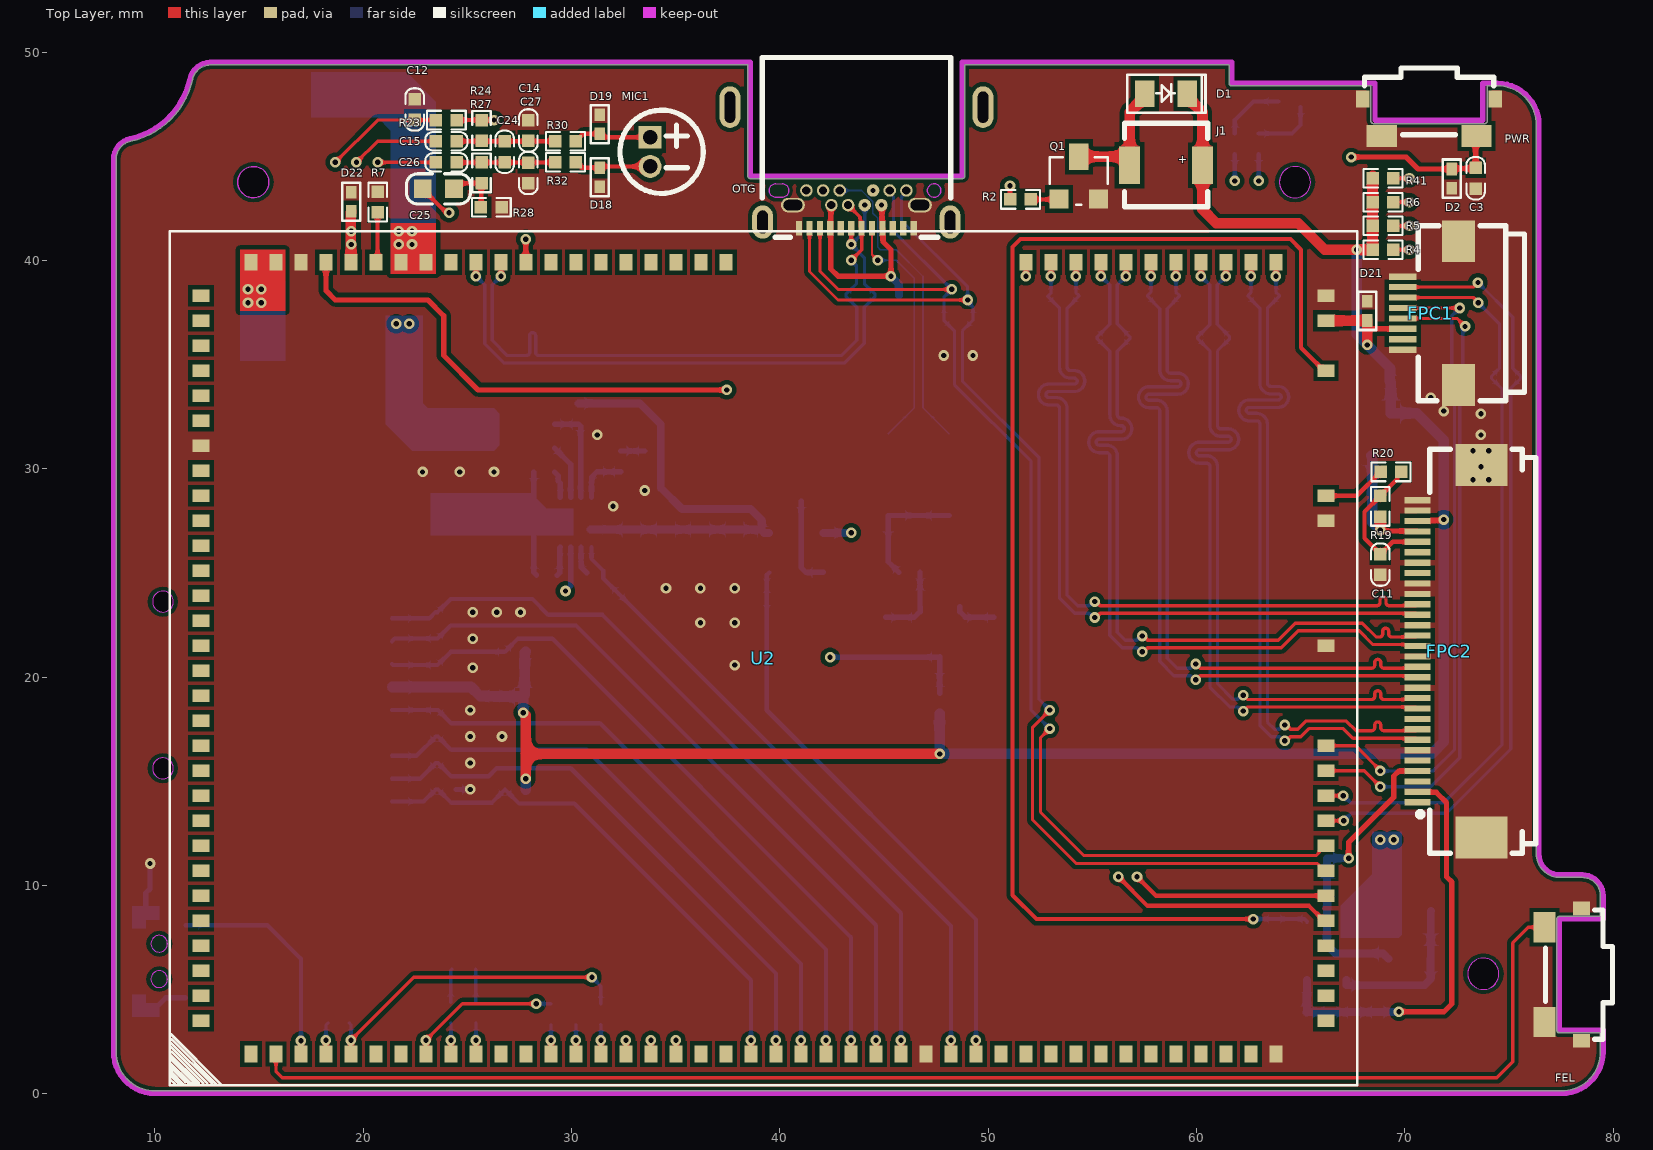
[diagram p0: Top Layer view]
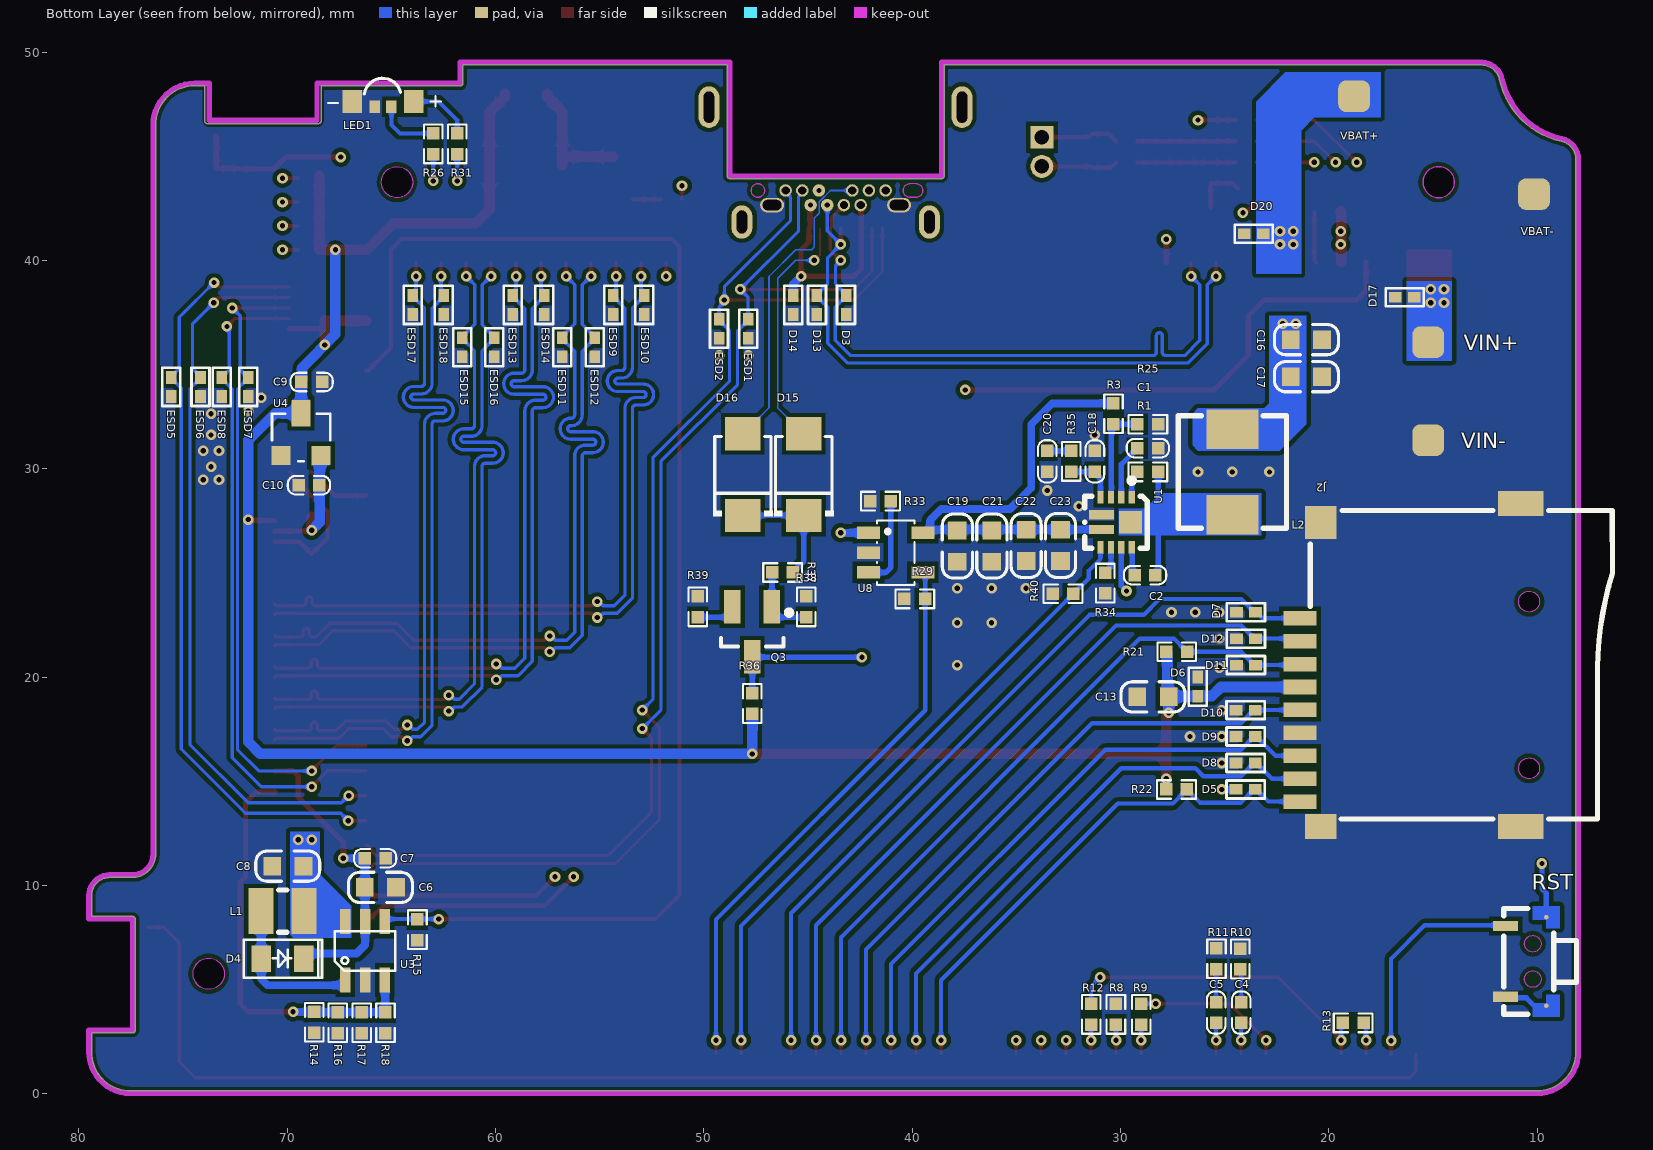
[diagram p1: Bottom Layer view, seen from below]
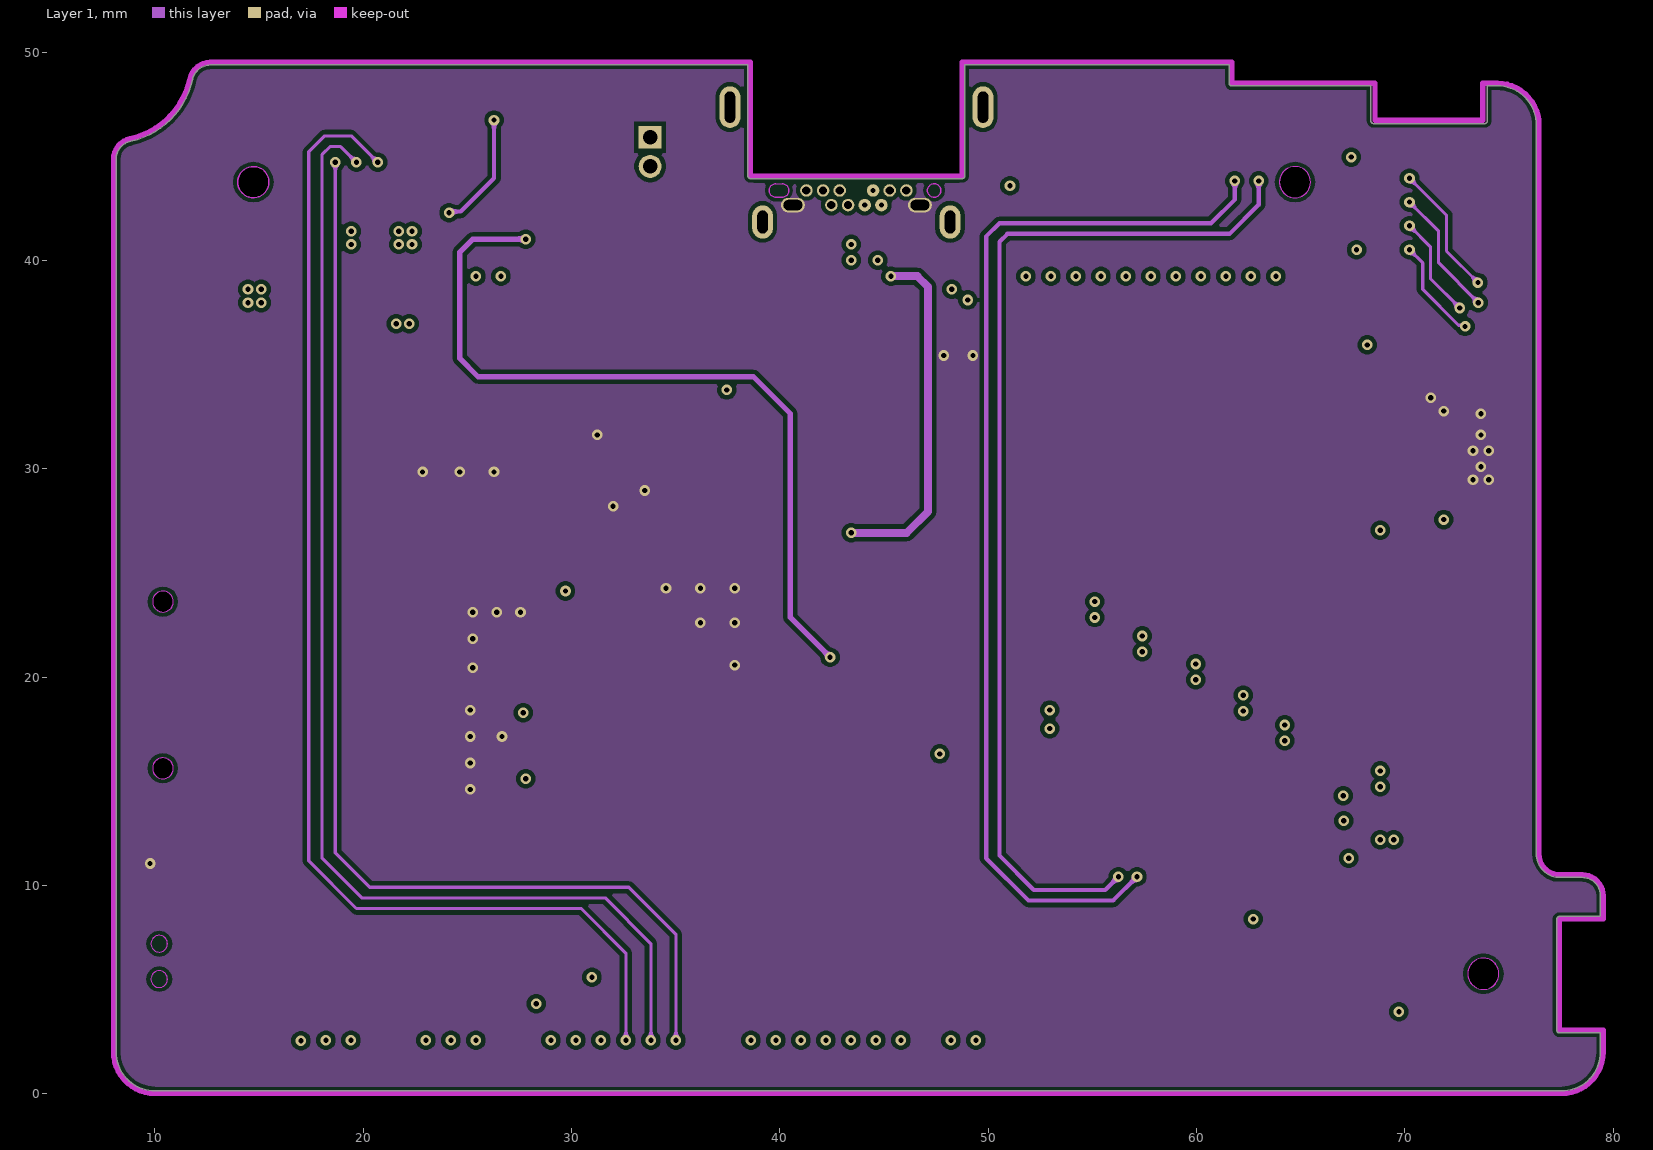
[diagram p2: Layer 1]
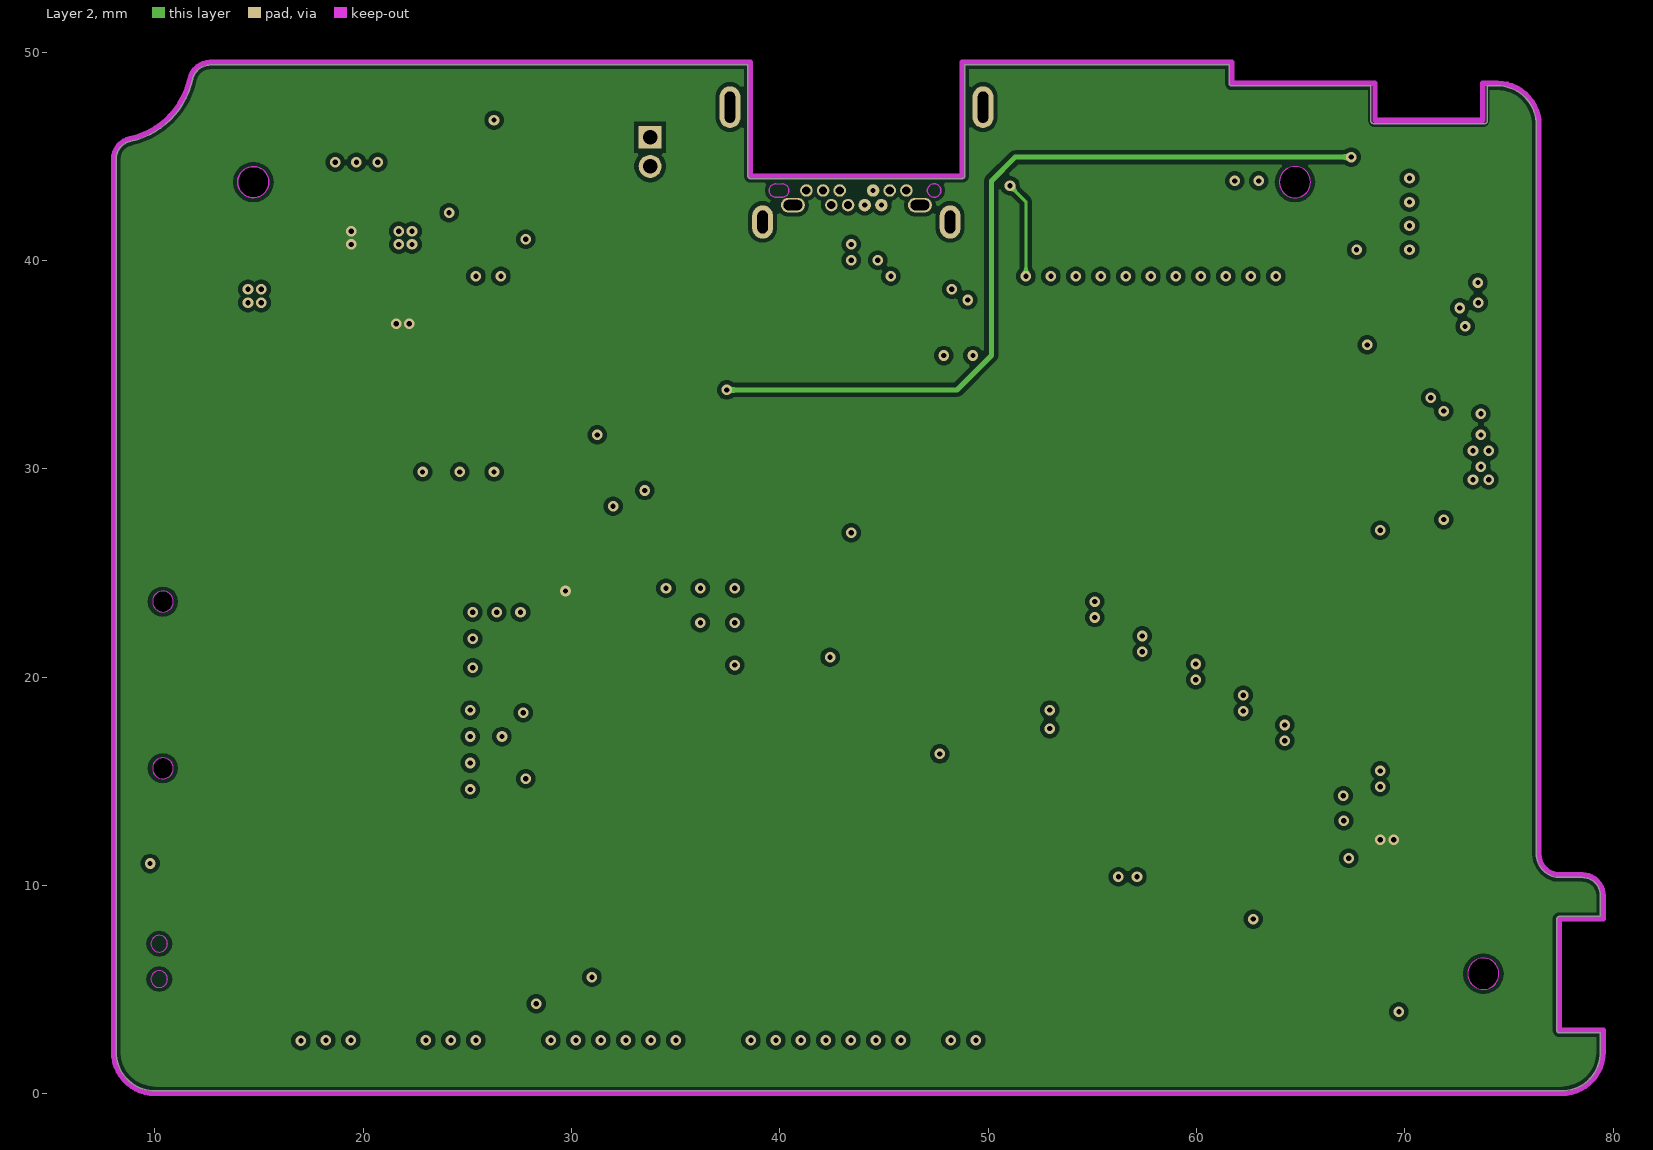
[diagram p3: Layer 2]
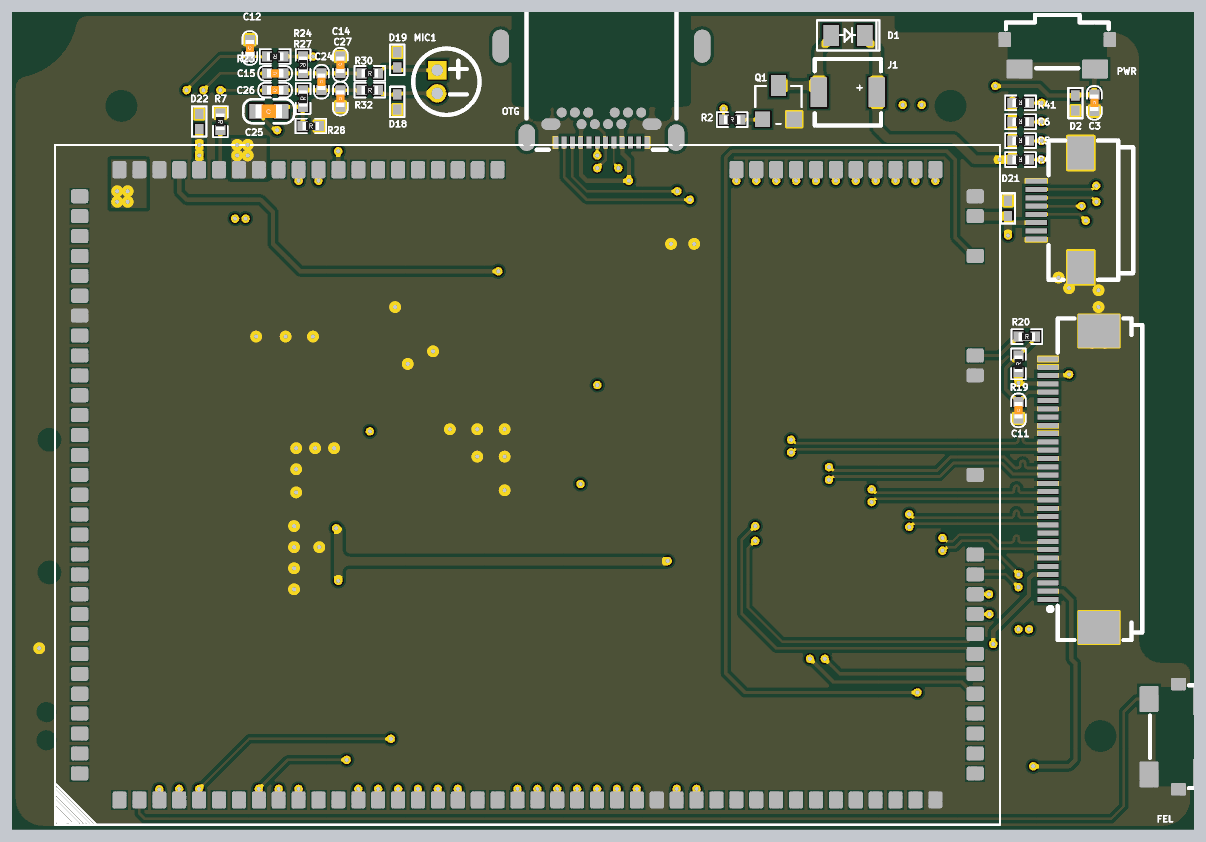
[diagram p4: 3D render of the assembled board from above, using the file's embedded part models]
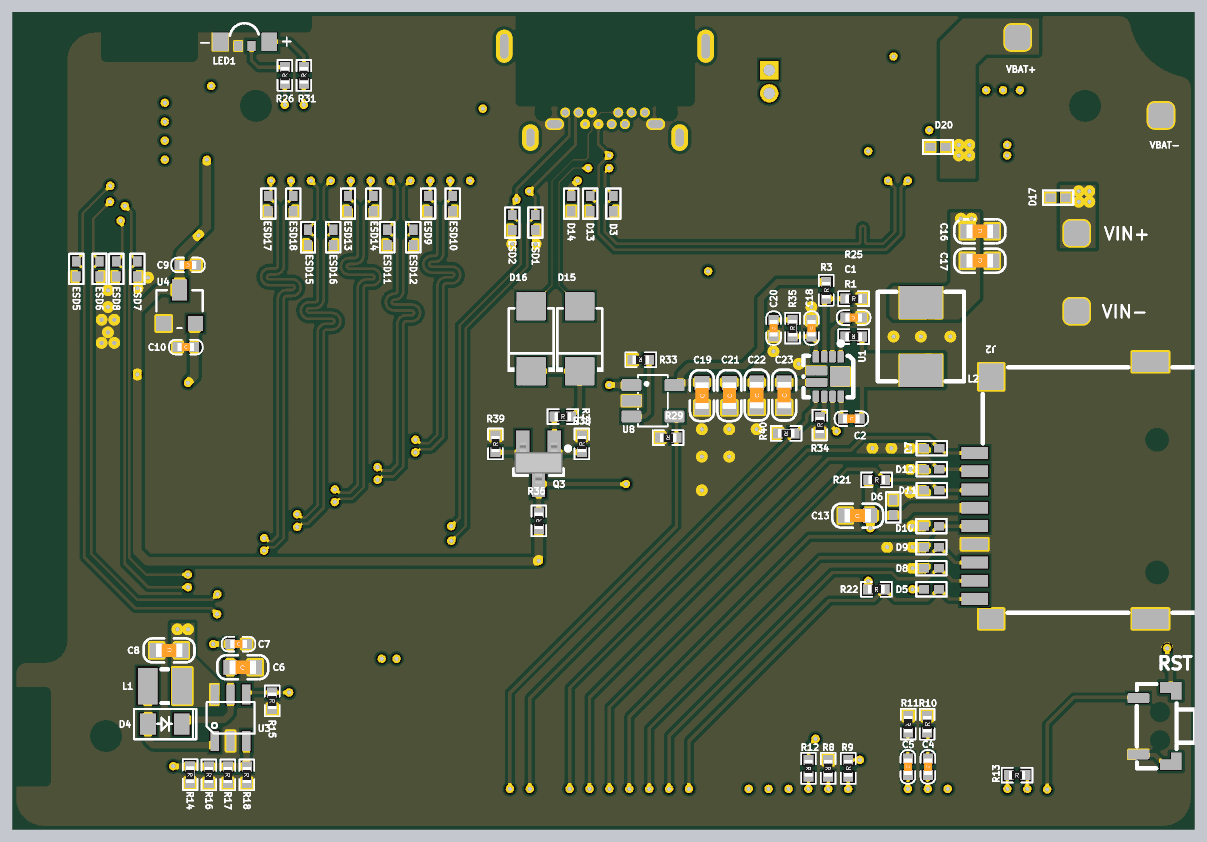
[diagram p5: 3D render of the assembled board from below, using the file's embedded part models]
# Altium PCB MISC105407.PcbDoc (part 1 of 2)
Units mm, origin at the board's own origin, x right, y up, seen from the top; angles counter-clockwise.
Board outline 71.25 x 49.25 mm, 4 copper layers (Top Layer, Layer 1, Layer 2, Bottom Layer), stack 0.603 mm thick; 129 components, 86 nets, 475 pads, 140 vias.

## Layer stack, top to bottom
Top Solder: solder mask 0.0102, Solder Resist, Dk 3.5
Top Layer: signal copper 0.0356
Dielectric 2: prepreg 0.0711, PP-006, Dk 4.1
Layer 1: signal copper 0.035
Dielectric 1: dielectric 0.32, FR-4, Dk 4.8
Layer 2: signal copper 0.035
Dielectric 3: prepreg 0.0711, PP-006, Dk 4.1
Bottom Layer: signal copper 0.0356
Bottom Solder: solder mask 0.0102, Solder Resist, Dk 3.5

## Board outline
8.154,2.006 ccw(c10.026,2.006) 10.026,0.134 77.526,0.134 ccw(c77.526,2.006) 79.399,2.006 79.399,2.921 77.43,2.921 cw(c77.43,3.048) 77.303,3.048 77.303,8.382 cw(c77.43,8.382) 77.43,8.509 79.399,8.509 79.399,9.506 ccw(c78.526,9.506) 78.526,10.379 77.446,10.379 cw(c77.446,11.506) 76.319,11.506 76.319,46.506 ccw(c74.446,46.506) 74.446,48.379 cw(c74.446,48.507) 74.445,48.379 73.965,48.379 73.965,46.696 cw(c73.838,46.696) 73.838,46.569 68.504,46.569 cw(c68.504,46.696) 68.376,46.696 68.376,48.379 61.696,48.379 cw(c61.696,48.506) 61.569,48.506 61.569,49.379 48.889,49.379 48.889,44.055 cw(c48.761,44.055) 48.761,43.927 48.606,43.927 cw(c48.538,44.035) 48.538,43.908 38.838,43.908 cw(c38.838,44.035) 38.77,43.927 38.601,43.927 cw(c38.601,44.055) 38.474,44.055 38.474,49.379 12.67,49.379 ccw(c12.67,53.145) 12.671,49.379 12.67,49.379 ccw(c12.67,48.506) 11.817,48.69 cw(c8.027,49.506) 8.843,45.716 cw(c8.596,46.862) 8.843,45.716 ccw(c8.827,45.791) 8.843,45.716 ccw(c9.027,44.862) 8.154,44.863
cut-out: 73.026,5.756 ccw(c73.776,5.756) 73.776,5.006 ccw(c73.776,5.756) 74.526,5.756 ccw(c73.776,5.756) 73.776,6.506 ccw(c73.776,5.756)
cut-out: 63.986,43.756 ccw(c64.736,43.756) 64.736,43.006 ccw(c64.736,43.756) 65.486,43.756 ccw(c64.736,43.756) 64.736,44.506 ccw(c64.736,43.756)
cut-out: 14.736,43.006 cw(c14.736,43.756) 13.986,43.756 cw(c14.736,43.756) 14.736,44.506 cw(c14.736,43.756) 15.486,43.756 cw(c14.736,43.756)

## Design rules (kind name [scope] priority, off if disabled: settings)
Clearance [All] p1: gap=0.051 ignorepadtopadclearanceinfootprint=FALSE except(0.203: Arc-Poly Track-Poly SMDPad-Poly THPad-Poly Via-Poly Fill-Poly Poly-Poly Poly-Region Poly-Text Poly-Hole)
ComponentClearance [All] p1: gap=0 collisioncheckmode=3 verticalgap=0 showdistances=FALSE
DiffPairsRouting [InDifferentialPairClass('D_90om')] p1: maxlimit=0.254 minlimit=0.203 mostfreqgap=0.203 toplayer_minwidth=0.158 toplayer_maxwidth=0.158 toplayer_prefwidth=0.158 midlayer1_minwidth=0.158 midlayer1_maxwidth=0.158 midlayer1_prefwidth=0.158 midlayer2_minwidth=0.158 midlayer2_maxwidth=0.158 midlayer2_prefwidth=0.158 bottomlayer_minwidth=0.158 bottomlayer_maxwidth=0.158 bottomlayer_prefwidth=0.158 maxuncoupledlength=12.7
MinimumSolderMaskSliver [All] p1: minsoldermaskwidth=0
PolygonConnect [All] p1: connectstyle=Direct reliefconductorwidth=0.254 reliefentries=4 polygonreliefangle="90 Angle" airgapwidth=0.254
RoutingVias [All] p1: holewidth=0.254 width=0.508 viastyle="Through Hole" minholewidth=0.254 minwidth=0.508 maxholewidth=0.254 maxwidth=0.508
SilkToSilkClearance [All] p1: silktosilkclearance=0
SilkToSolderMaskClearance [IsPad] p1: minsilkscreentomaskgap=0 clearancetoexposedcopper=TRUE
SolderMaskExpansion [All] p1: expansion=0.102 istentingtop=FALSE
Width [All] p1: maxlimit=1.27 minlimit=0.025 preferedwidth=0.254
25 further rules are at their usual default settings.

## Classes and differential pairs
differential pair class D_90om: MICIN1 MIPI_CL MIPI_D0 MIPI_D1 MIPI_D2 MIPI_D3 USB0
differential pair MICIN1: +MICIN1_P -MICIN1_N
differential pair MIPI_D3: +MIPI_D3_P -MIPI_D3_N
differential pair MIPI_D2: +MIPI_D2_P -MIPI_D2_N
differential pair MIPI_D1: +MIPI_D1_P -MIPI_D1_N
differential pair MIPI_CL: +MIPI_CL_P -MIPI_CL_N
differential pair USB0: +USB0_P -USB0_N
differential pair MIPI_D0: +MIPI_D0_P -MIPI_D0_N

## Components (designator, comment, footprint, x,y, rotation, side; value= is the part's Value field where it differs from the comment)
C1 "C-16-225(±10%)" C0402 28.694,30.988 r180 bottom
C2 "C-50-104(±10%)" C0402 28.829,24.892 r0 bottom
C3 "C-25-104" C0402 73.406,43.942 r90 top
C4 "C-25-104" C0402 24.212,3.896 r270 bottom
C5 "C-25-104" C0402 25.418,3.896 r270 bottom
C6 "C-25-106" C0603 65.532,9.906 r180 bottom
C7 "C-25-104" C0402 65.786,11.303 r0 bottom
C8 "C-25-106" C0603 69.977,10.922 r0 bottom
C9 "C-25-104" C0402 68.834,34.163 r180 bottom
C10 "C-25-104" C0402 68.961,29.21 r0 bottom
C11 "C-25-104" C0402 68.834,25.4 r270 top
C12 "C-50-105" C0402 22.479,47.244 r270 top
C13 "C-25-106" C0603 28.448,19.05 r180 bottom
C14 "C-50-330" C0402 27.94,46.236 r270 top
C15 "C-50-104" C0402 24.003,45.72 r0 top
C16 "C-16-106(±10%)" C0603 21.082,36.195 r0 bottom
C17 "C-16-106(±10%)" C0603 21.082,34.417 r0 bottom
C18 "C-50-472(±10%)" C0402 31.234,30.353 r270 bottom
C19 "C-16-106(±10%)" C0603 37.838,26.289 r90 bottom
C20 "C-50-220(±10%)" C0402 33.52,30.353 r90 bottom
C21 "C-16-106(±10%)" C0603 36.187,26.289 r90 bottom
C22 "C-16-106(±10%)" C0603 34.536,26.32 r90 bottom
C23 "C-16-106(±10%)" C0603 32.885,26.32 r90 bottom
C24 "C-50-101" C0402 26.797,45.212 r90 top
C25 "C-50-106" C0603 23.622,43.434 r0 top
C26 "C-50-104" C0402 24.003,44.704 r0 top
C27 "C-50-330" C0402 27.94,44.196 r90 top
D1 "1N5819" SOD323 58.547,48.006 r0 top
D2 "AU0511P1" ESD0402A 72.263,43.942 r90 top
D3 "AU0511P1" ESD0402A 43.18,37.846 r270 bottom
D4 "1N5819" SOD323 70.231,6.477 r180 bottom
D5 "AU0511P1" ESD0402A 24.019,14.604 r0 bottom
D6 "AU0511P1" ESD0402A 26.305,19.557 r90 bottom
D7 "AU0511P1" ESD0402A 24.003,23.114 r0 bottom
D8 "AU0511P1" ESD0402A 24.019,15.874 r0 bottom
D9 "AU0511P1" ESD0402A 24.019,17.144 r0 bottom
D10 "AU0511P1" ESD0402A 24.019,18.414 r0 bottom
D11 "AU0511P1" ESD0402A 24.003,20.574 r0 bottom
D12 "AU0511P1" ESD0402A 24.003,21.844 r0 bottom
D13 "AU0511P1" ESD0402A 44.577,37.846 r270 bottom
D14 "AU0511P1" ESD0402A 45.72,37.846 r270 bottom
D15 "SS34F_C18199199" SMAF_L3.5-W2.6-LS4.7-RD-1 45.212,29.718 r90 bottom
D16 "SS34F_C18199199" SMAF_L3.5-W2.6-LS4.7-RD-1 48.133,29.718 r90 bottom
D17 "AU0511P1" ESD0402A 16.383,38.227 r0 bottom
D18 "AU0511P1" ESD0402A 31.368,44.009 r90 top
D19 "AU0511P1" ESD0402A 31.37,46.517 r270 top
D20 "AU0511P1" ESD0402A 23.622,41.275 r0 bottom
D21 "AU0511P1" ESD0402A 68.199,37.592 r90 top
D22 "AU0511P1" ESD0402A 19.431,42.799 r270 top
ESD1 "AU0511P1" ESD0402A 47.879,36.703 r270 bottom
ESD2 "AU0511P1" ESD0402A 49.276,36.703 r270 bottom
ESD5 "AU0511P1" ESD0402A 75.565,33.909 r270 bottom
ESD6 "AU0511P1" ESD0402A 74.168,33.909 r270 bottom
ESD7 "AU0511P1" ESD0402A 71.882,33.909 r270 bottom
ESD8 "AU0511P1" ESD0402A 73.152,33.909 r270 bottom
ESD9 "AU0511P1" ESD0402A 54.356,37.846 r270 bottom
ESD10 "AU0511P1" ESD0402A 52.873,37.846 r270 bottom
ESD11 "AU0511P1" ESD0402A 56.81,35.814 r270 bottom
ESD12 "AU0511P1" ESD0402A 55.245,35.814 r270 bottom
ESD13 "AU0511P1" ESD0402A 59.182,37.846 r270 bottom
ESD14 "AU0511P1" ESD0402A 57.658,37.846 r270 bottom
ESD15 "AU0511P1" ESD0402A 61.595,35.814 r270 bottom
ESD16 "AU0511P1" ESD0402A 60.071,35.814 r270 bottom
ESD17 "AU0511P1" ESD0402A 63.982,37.846 r270 bottom
ESD18 "AU0511P1" ESD0402A 62.484,37.846 r270 bottom
FEL "TSB017A3126A02" KEY-SMD_YTSB017A0312502B#1 77.597,5.715 r90 top
FPC1 "AFC01-S08FCA-00" FPC-SMD_P0.50-8P_FGS-XJ-H2.0 71.247,37.465 r270 top locked
FPC2 "FPC-05F-30PH20" FPC-SMD_30P-P0.50_XUNPU_FPC-05F-30PH20 72.147,21.241 r90 top locked
J1 "FUET-4020" BUZ-SMD_L4.0-W4.0-P3.50-L 58.547,44.577 r180 top
J2 "TF-115-BCP9" TF-SMD_TF-115-BCP9 16.095,20.571 r90 bottom locked
L1 "10uH" IND-SMD_L2.5-W2.0 70.231,8.763 r180 bottom
L2 "FXL0518-2R2-M" IND-SMD_L5.2-W5.4 24.638,29.845 r270 bottom
LED1 "XL-3210SURUGC" LED-SMD_4P-L3.2-W1.5_HTG-3210SURUBGC 65.405,47.498 r180 bottom
MIC1 "GMI4015P-2C-64db" MIC-TH_BD4.0-P1.40-D0.4-L-FD 33.782,45.212 r270 top
OTG "GT-USB-9009B" USB-C-SMD_GT-USB-9009B 43.688,44.45 r180 top (schematic designator USBC1)
PWR "TSB017A3126A02" KEY-SMD_YTSB017A0312502B#2 71.171,46.863 r180 top
Q1 "S9013" SOT23 54.356,43.942 r0 top
Q3 "8050-S" SOT-23-3 46.741,23.368 r270 bottom
R1 "R-304J" R0402 28.694,29.845 r0 bottom
R2 "R-152J" R0402 51.562,42.926 r0 top
R3 "R-304F" R0402 30.345,32.639 r90 bottom
R4 "R-472J" R0402 68.961,40.513 r180 top
R5 "R-472J" R0402 68.961,41.656 r180 top
R6 "R-472J" R0402 68.961,42.799 r180 top
R7 "R-103J" R0402 20.701,42.799 r270 top
R8 "R-0J" R0402 30.226,3.81 r270 bottom
R9 "R-202J" R0402 29.019,3.81 r90 bottom
R10 "R-220J" R0402 24.257,6.469 r90 bottom
R11 "R-220J" R0402 25.4,6.477 r270 bottom
R12 "R-105J" R0402 31.414,3.81 r270 bottom
R13 "R-104J" R0402 18.84,3.397 r180 bottom
R14 "NC" R0402 68.707,3.429 r270 bottom
R15 "1M" R0402 63.754,7.874 r270 bottom
R16 "8R2" R0402 67.574,3.408 r270 bottom
R17 "8R2" R0402 66.431,3.408 r270 bottom
R18 "8R2" R0402 65.288,3.408 r270 bottom
R19 "R-103J" R0402 68.834,28.194 r90 top
R20 "R-0J" R0402 69.342,29.845 r0 top
R21 "R-103J" R0402 27.305,21.209 r180 bottom
R22 "R-103J" R0402 27.321,14.604 r180 bottom
R23 "R-102" R0402 24.003,46.736 r180 top
R24 "R-152" R0402 25.689,46.236 r270 top
R25 "R-104F" R0402 28.694,32.131 r180 bottom
R26 "R-202J" R0402 62.992,45.593 r90 bottom
R27 "R-152" R0402 25.689,44.2 r90 top
R28 "R-102" R0402 26.162,42.545 r0 top
R29 "R-103J" R0402 39.878,23.749 r0 bottom
R30 "R-104F" R0402 29.718,45.72 r0 top
R31 "R-202J" R0402 61.849,45.593 r90 bottom
R32 "R-304F" R0402 29.718,44.704 r0 top
R33 "R-332J" R0402 41.529,28.448 r0 bottom
R34 "R-154J" R0402 30.734,24.511 r90 bottom
R35 "R-622F" R0402 32.377,30.353 r90 bottom
R36 "R-103J" R0402 47.678,18.729 r90 bottom
R37 "R-103J" R0402 46.228,25.019 r180 bottom
R38 "R-103J" R0402 45.085,23.368 r90 bottom
R39 "R-5R0J" R0402 50.292,23.368 r90 bottom
R40 "R-103J" R0402 32.766,24.003 r0 bottom
R41 "R-472J" R0402 68.961,43.942 r180 top
RST "LXTD-0204-034" SW-SMD_LXTD-0204-034 10.541,6.35 r90 bottom
U1 "TPS61089RNRR" VQFN-HR_L2.5-W2.0-P0.50-TL-EP 30.218,27.432 r270 bottom
U2 "HelperA133Core" "A133 - duplicate" 10.743,0.385 r90 top locked
U3 "HM5663" SOT23-6 66.04,6.858 r270 bottom
U4 "xc6206p182mr" SOT23 69.342,31.623 r180 bottom
U8 "MT9700" SOT-23-5_L3.0-W1.7-P0.95-LS2.8-BR 40.797,25.974 r0 bottom
VBAT+ "Header 1" HDR-LI-1P 18.796,47.879 r90 bottom
VBAT- "Header 1" HDR-LI-1P 10.16,43.18 r90 bottom
VIN+ "Header 1" HDR-LI-1P 15.24,36.068 r90 bottom
VIN- "Header 1" HDR-LI-1P 15.24,31.369 r90 bottom

## Footprints (in the part's own frame and the unit in brackets; to place one, negate y for a bottom-side part, rotate by r counter-clockwise, add the part's x,y. Pads: shape width x height; smd on the part's side, far side on the other; paste and mask are expansions set on the pad)
"A133 - duplicate" [mil]
  rect 31.5x24 smd paste+4.73: 1(59.83,-152.68) 2(59.83,-199.92) 3(59.83,-247.17) 4(59.83,-294.41) 5(59.83,-341.65) 6(59.83,-388.9) 7(59.83,-436.14) 8(59.83,-483.39) 9(59.83,-530.63) 10(59.83,-577.87) 11(59.83,-625.12) 12(59.83,-672.36) 13(59.83,-719.61) 14(59.83,-766.85) 15(59.83,-814.09) 16(59.83,-861.34) 17(59.83,-908.58) 18(59.83,-955.83) 19(59.83,-1003.07) 20(59.83,-1050.32) 21(59.83,-1097.56) 22(59.83,-1144.8) 23(59.83,-1192.05) 24(59.83,-1239.29) 25(59.83,-1286.54) 26(59.83,-1333.78) 27(59.83,-1381.02) 28(59.83,-1428.27) 29(59.83,-1475.51) 30(59.83,-1522.76) 31(59.83,-1570) 32(59.83,-1617.24) 33(59.83,-1664.49) 34(59.83,-1711.73) 35(59.83,-1758.98) 36(59.83,-1806.22) 37(59.83,-1853.46) 38(59.83,-1900.71) 39(59.83,-1947.95) 40(59.83,-1995.2) 41(59.83,-2042.44) 42(59.83,-2089.68) 73(1555.89,-2089.68) 74(1555.89,-2042.44) 75(1555.89,-1995.2) 76(1555.89,-1947.95) 77(1555.89,-1900.71) 78(1555.89,-1853.46) 79(1555.89,-1806.22) 80(1555.89,-1758.98) 81(1555.89,-1711.73) 82(1555.89,-1664.49) 83(1555.89,-1617.24) 95(1555.89,-1050.32) 96(1555.89,-1003.07) 97(1555.89,-955.83) 98(1555.89,-908.58) 99(1555.89,-861.34) 100(1555.89,-814.09) 101(1555.89,-766.85) 102(1555.89,-719.61) 103(1555.89,-672.36) 104(1555.89,-625.12) 105(1555.89,-577.87) 106(1555.89,-530.63) 107(1555.89,-483.39) 108(1555.89,-436.14) 109(1555.89,-388.9) 110(1555.89,-341.65) 111(1555.89,-294.41) 112(1555.89,-247.17) 113(1555.89,-199.92) 114(1555.89,-152.68)
  rect 24x31.5 smd paste+4.73: 43(122.82,-2184.17) 44(170.06,-2184.17) 45(217.31,-2184.17) 46(264.55,-2184.17) 47(311.8,-2184.17) 48(359.04,-2184.17) 49(406.28,-2184.17) 50(453.53,-2184.17) 51(500.77,-2184.17) 52(548.02,-2184.17) 53(595.26,-2184.17) 54(642.5,-2184.17) 58(831.48,-2184.17) 63(1067.7,-2184.17) 64(1114.94,-2184.17) 69(1351.17,-2184.17) 71(1445.65,-2184.17) 72(1492.9,-2184.17) 115(1492.9,-58.19) 116(1445.65,-58.19) 117(1398.41,-58.19) 118(1351.17,-58.19) 119(1303.92,-58.19) 120(1256.68,-58.19) 121(1209.43,-58.19) 122(1162.19,-58.19) 123(1114.94,-58.19) 124(1067.7,-58.19) 125(1020.46,-58.19) 126(973.21,-58.19) 127(925.97,-58.19) 128(878.72,-58.19) 129(831.48,-58.19) 130(784.24,-58.19) 131(736.99,-58.19) 132(689.75,-58.19) 133(642.5,-58.19) 134(595.26,-58.19) 135(548.02,-58.19) 136(500.77,-58.19) 137(453.53,-58.19) 138(406.28,-58.19) 139(359.04,-58.19) 140(311.8,-58.19) 141(264.55,-58.19) 142(217.31,-58.19) 143(170.06,-58.19) 144(122.82,-58.19)
  silkscreen extent 1,-2243 1615,1
BUZ-SMD_L4.0-W4.0-P3.50-L [mm]
  rect 1x1.8 smd: 1(-1.75,0) 2(1.75,0)
  silkscreen extent -2,-2 2,2
C0402 [mm]
  rect 0.6x0.6 smd: 1(0.5,0) 2(-0.5,0)
  silkscreen extent -1.02,-0.44 1.02,0.44, body extent -0.5,-0.25 0.5,0.25, height 0.49
C0603 [mm]
  rect 0.85x0.9 smd: 1(-0.75,0) 2(0.75,0)
  silkscreen extent -1.54,-0.72 1.54,0.72, body extent -0.8,-0.41 0.8,0.4, height 0.88
ESD0402A [mil]
  rect 24x20 smd: 1(-18.63,-0.06) 2(17.37,-0.06)
  silkscreen extent -37,-17 35,17
FPC-SMD_30P-P0.50_XUNPU_FPC-05F-30PH20 [mm]
  rect 0.3x1.25 smd paste+0 mask+0.05: 1(-7.25,1.538) 2(-6.75,1.538) 3(-6.25,1.538) 4(-5.75,1.538) 5(-5.25,1.538) 6(-4.75,1.538) 7(-4.25,1.538) 8(-3.75,1.538) 9(-3.25,1.538) 10(-2.75,1.538) 11(-2.25,1.538) 12(-1.75,1.538) 13(-1.25,1.538) 14(-0.75,1.538) 15(-0.25,1.538) 16(0.25,1.538) 17(0.75,1.538) 18(1.25,1.538) 19(1.75,1.538) 20(2.25,1.538) 21(2.75,1.538) 22(3.25,1.538) 23(3.75,1.538) 24(4.25,1.538) 25(4.75,1.538) 26(5.25,1.538) 27(5.75,1.538) 28(6.25,1.538) 29(6.75,1.538) 30(7.25,1.538)
  rect 2x2.5 smd paste+0 mask+0.05: 31(8.94,-1.538) 32(-8.94,-1.538)
  silkscreen extent -9.7,-4.15 9.7,1.53
FPC-SMD_P0.50-8P_FGS-XJ-H2.0 [mm]
  rect 0.3x1.3 smd paste+0 mask+0.05: 1(1.75,-1.34) 2(1.25,-1.34) 3(0.75,-1.34) 4(0.25,-1.34) 5(-0.25,-1.34) 6(-0.75,-1.34) 7(-1.252,-1.338) 8(-1.75,-1.34)
  rect 2x1.6 smd: 9(3.45,1.34) 10(-3.45,1.34)
  silkscreen extent -4.2,-0.6 4.2,4.5
HDR-LI-1P [mil]
  rrect50% 60x60 smd: 1(0,0)
IND-SMD_L2.5-W2.0 [mm]
  rect 1.2x2.2 smd: 1(1.028,0) 2(-1.028,0)
  silkscreen extent -0.2,-1.02 0.2,1.02
IND-SMD_L5.2-W5.4 [mm]
  rect 1.9x2.5 smd paste+0.051: 1(-2.05,0) 2(2.05,0)
  silkscreen extent -2.7,-2.6 2.7,2.6
KEY-SMD_YTSB017A0312502B#1 [mm]
  rect 1.45x1.05 smd paste+0.051 mask+0: 1(-2.275,0.887) 2(2.275,0.887)
  rect 0.65x0.8 smd paste+0.051 mask+0: 3(-3.175,-0.887) 4(3.175,-0.887)
  Keep-Out Layer lines w0.254: -2.667,0.167 2.667,0.167 ; -2.667,0.167 -2.667,-1.93 -2.667,0.167 ; -2.667,0.167 2.667,0.167 ; 2.667,0.167 2.667,-1.93 2.667,0.167
  silkscreen extent -3.1,-2.38 3.1,0.84
KEY-SMD_YTSB017A0312502B#2 [mm]
  rect 1.45x1.05 smd paste+0.051 mask+0: 1(-2.275,0.887) 2(2.275,0.887)
  rect 0.65x0.8 smd paste+0.051 mask+0: 3(-3.175,-0.887) 4(3.175,-0.887)
  silkscreen extent -3.1,-2.38 3.1,0.84
LED-SMD_4P-L3.2-W1.5_HTG-3210SURUBGC [mm]
  rect 0.5x0.6 smd paste+0 mask+0.05: 1(0.4,-0.132) 2(-0.4,-0.132)
  rect 0.95x1.1 smd paste+0 mask+0.05: 3(1.475,0.132) 4(-1.475,0.132)
  silkscreen extent -2.64,-0.12 2.77,1.24
MIC-TH_BD4.0-P1.40-D0.4-L-FD [mm]
  rect 1.1x1.1 hole 0.7 paste+0.051: 1(-0.7,0)
  round 1.1 hole 0.7 paste+0.051: 2(0.7,0)
  silkscreen extent -2,-1.45 2,2.55
R0402 [mm] "Chip Capacitor; Body 1.0 x 0.5 mm (LxW typ)"
  rect 0.6x0.6 smd: 1(-0.5,0) 2(0.5,0)
  silkscreen extent -0.93,-0.44 0.93,0.44, body extent -0.5,-0.25 0.5,0.25, height 0.38
SMAF_L3.5-W2.6-LS4.7-RD-1 [mm]
  rect 1.6x1.7 smd paste+0.051: 1(-1.96,0) 2(1.96,0)
  silkscreen extent -2.01,-1.43 1.83,1.42
SOD323 [mil]
  rect 37x50 smd: 1(-40,0) 2(40,0)
  silkscreen extent -73,-36 75,36
SOT23 [mil]
  rect 36x36 smd: 1(-37.5,-39) 2(37.5,-39)
  rect 36x50 smd: 3(0,41)
  silkscreen extent -55,-50 55,40
SOT23-6 [mm]
  rect 1.2x0.5 smd: 1(1.4,-1.177) 2(1.4,-0.227) 3(1.4,0.723) 4(-1.4,0.723) 5(-1.4,-0.227) 6(-1.4,-1.177)
  silkscreen extent -0.95,-1.68 0.95,1.22
SOT-23-3 [mm]
  rect 1.6x0.8 smd: 1(0,0) 2(0,-1.9) 3(2.4,-0.95)
  silkscreen extent 0.15,-2.45 1.9,0.95, body extent -0.11,-2.39 2.39,0.5, height 1.07
SOT-23-5_L3.0-W1.7-P0.95-LS2.8-BR [mm]
  rect 1.1x0.6 smd paste+0.051: 1(1.3,-0.95) 2(1.3,0) 3(1.3,0.95) 4(-1.3,0.95) 5(-1.3,-0.95)
  silkscreen extent -0.9,-1.55 0.9,1.55
SW-SMD_LXTD-0204-034 [mm]
  rect 0.5x1.2 smd paste+0.051: 1(-1.7,0.975) 2(1.7,0.975)
  round 0.21 smd: 3(2.125,-0.975) 4(-2.125,-0.975)
  Top Layer region: 2.65,-0.325 2.65,-0.975 2.65,-1.625 2,-1.625 1.6,-1.625 1.6,-0.975 2,-0.975 2,-0.325 2.65,-0.325
  Top Layer region: -2.65,-0.325 -2.65,-0.975 -2.65,-1.625 -2,-1.625 -1.6,-1.625 -1.6,-0.975 -2,-0.975 -2,-0.325 -2.65,-0.325
  Keep-Out Layer circle w0.003: c0.85,-0.325 r0.4
  Keep-Out Layer circle w0.003: c-0.85,-0.325 r0.4
  Keep-Out Layer region: 1.25,-0.325 1.21,-0.499 1.099,-0.638 0.939,-0.715 0.761,-0.715 0.6,-0.638 0.489,-0.499 0.45,-0.325 0.45,-0.325 0.489,-0.151 0.6,-0.012 0.761,0.065 0.939,0.065 1.099,-0.012 1.21,-0.151 1.25,-0.325
  Keep-Out Layer region: 1.25,-0.325 1.21,-0.499 1.099,-0.638 0.939,-0.715 0.761,-0.715 0.6,-0.638 0.489,-0.499 0.45,-0.325 0.45,-0.325 0.489,-0.151 0.6,-0.012 0.761,0.065 0.939,0.065 1.099,-0.012 1.21,-0.151 1.25,-0.325
  Keep-Out Layer region: -0.45,-0.325 -0.49,-0.499 -0.601,-0.638 -0.761,-0.715 -0.939,-0.715 -1.099,-0.638 -1.21,-0.499 -1.25,-0.325 -1.25,-0.325 -1.21,-0.151 -1.099,-0.012 -0.939,0.065 -0.761,0.065 -0.601,-0.012 -0.49,-0.151 -0.45,-0.325
  Keep-Out Layer region: -0.45,-0.325 -0.49,-0.499 -0.601,-0.638 -0.761,-0.715 -0.939,-0.715 -1.099,-0.638 -1.21,-0.499 -1.25,-0.325 -1.25,-0.325 -1.21,-0.151 -1.099,-0.012 -0.939,0.065 -0.761,0.065 -0.601,-0.012 -0.49,-0.151 -0.45,-0.325
  silkscreen extent -2.54,-2.43 2.54,1.07
TF-SMD_TF-115-BCP9 [mm]
  rect 0.7x1.6 smd: 1(2.25,5.3) 2(1.15,5.3) 3(0.05,5.3) 4(-1.05,5.3) 5(-2.15,5.3) 6(-3.25,5.3) 7(-4.35,5.3) 8(-5.45,5.3) 9(-6.55,5.3)
  rect 1.2x1.5 smd: 10(-7.75,4.3)
  rect 1.2x2.2 smd: 11(-7.75,-5.3) 13(7.75,-5.3)
  rect 1.6x1.5 smd: 12(6.85,4.3)
  Keep-Out Layer board cut-out: -4.45,-5.7 -4.499,-5.917 -4.638,-6.091 -4.839,-6.187 -5.061,-6.187 -5.262,-6.091 -5.4,-5.917 -5.45,-5.7 -5.45,-5.7 -5.4,-5.483 -5.262,-5.309 -5.061,-5.213 -4.839,-5.213 -4.638,-5.309 -4.499,-5.483 -4.45,-5.7
  Keep-Out Layer board cut-out: 3.55,-5.7 3.501,-5.917 3.362,-6.091 3.161,-6.187 2.939,-6.187 2.738,-6.091 2.6,-5.917 2.55,-5.7 2.55,-5.7 2.6,-5.483 2.738,-5.309 2.939,-5.213 3.161,-5.213 3.362,-5.309 3.501,-5.483 3.55,-5.7
  Keep-Out Layer circle w0.025: c-4.95,-5.7 r0.5
  Keep-Out Layer circle w0.025: c3.05,-5.7 r0.5
  Keep-Out Layer region: -4.45,-5.7 -4.499,-5.917 -4.638,-6.091 -4.839,-6.187 -5.061,-6.187 -5.262,-6.091 -5.4,-5.917 -5.45,-5.7 -5.45,-5.7 -5.4,-5.483 -5.262,-5.309 -5.061,-5.213 -4.839,-5.213 -4.638,-5.309 -4.499,-5.483 -4.45,-5.7
  Keep-Out Layer region: 3.55,-5.7 3.501,-5.917 3.362,-6.091 3.161,-6.187 2.939,-6.187 2.738,-6.091 2.6,-5.917 2.55,-5.7 2.55,-5.7 2.6,-5.483 2.738,-5.309 2.939,-5.213 3.161,-5.213 3.362,-5.309 3.501,-5.483 3.55,-5.7
  silkscreen extent -7.38,-9.7 7.42,4.81
USB-C-SMD_GT-USB-9009B [mm]
  oval 1x1.6 hole 0.5 slot 1.1 at 90 deg paste+0.051 mask+0: 2(4.505,2.605) 5(-4.495,2.605)
  oval 1x2 hole 0.5 slot 1.5 at 90 deg paste+0.051 mask+0: 3(6.075,-2.905) 4(-6.075,-2.905)
  rect 0.3x0.7 smd paste-100 mask+0.051: A1(-2.745,2.905) A2(-2.245,2.905) A3(-1.745,2.905) A4(-1.245,2.905) A5(-0.745,2.905) A6(-0.245,2.905) A7(0.255,2.905) A8(0.755,2.905) A9(1.255,2.905) A10(1.755,2.905) A11(2.255,2.905) A12(2.755,2.905)
  oval 1.15x0.7 hole 0.5 slot 0.9 at 0 deg paste+0.051 mask+0: B1(3.055,1.795) B12(-3.045,1.795)
  round 0.6 hole 0.4 paste+0.051 mask+0: B2(2.405,1.095) B3(1.605,1.095) B4(1.205,1.795) B5(0.805,1.095) B6(0.405,1.795) B10(-1.595,1.095) B11(-2.395,1.095)
  round 0.6 hole 0.25 paste+0.051 mask+0: B7(-0.395,1.795) B8(-0.795,1.095) B9(-1.195,1.795)
  Keep-Out Layer circle w0.003: c-3.725,1.095 r0.325
  Keep-Out Layer region: -3.4,1.095 -3.432,0.954 -3.522,0.841 -3.653,0.778 -3.797,0.778 -3.928,0.841 -4.018,0.954 -4.05,1.095 -4.05,1.095 -4.018,1.236 -3.928,1.349 -3.797,1.412 -3.653,1.412 -3.522,1.349 -3.432,1.236 -3.4,1.095
  Keep-Out Layer region: -3.4,1.095 -3.432,0.954 -3.522,0.841 -3.653,0.778 -3.797,0.778 -3.928,0.841 -4.018,0.954 -4.05,1.095 -4.05,1.095 -4.018,1.236 -3.928,1.349 -3.797,1.412 -3.653,1.412 -3.522,1.349 -3.432,1.236 -3.4,1.095
  Keep-Out Layer region: 3.575,1.42 3.875,1.42 4.016,1.388 4.129,1.298 4.192,1.167 4.192,1.023 4.129,0.892 4.016,0.802 3.875,0.77 3.875,0.77 3.575,0.77 3.434,0.802 3.321,0.892 3.258,1.023 3.258,1.167 3.321,1.298 3.434,1.388 3.575,1.42
  Keep-Out Layer region: 3.575,1.42 3.875,1.42 4.016,1.388 4.129,1.298 4.192,1.167 4.192,1.023 4.129,0.892 4.016,0.802 3.875,0.77 3.875,0.77 3.575,0.77 3.434,0.802 3.321,0.892 3.258,1.023 3.258,1.167 3.321,1.298 3.434,1.388 3.575,1.42
  Keep-Out Layer lines w0.003: 3.875,1.42 cw(c3.875,1.095) 3.875,0.77 3.575,0.77 cw(c3.575,1.095) 3.575,1.42 3.875,1.42
  silkscreen extent -4.52,-5.29 4.52,3.34
VQFN-HR_L2.5-W2.0-P0.50-TL-EP [mm]
  rect 0.6x0.3 smd paste+0.051: 1(-1.199,0.75) 2(-1.199,0.25) 3(-1.199,-0.25) 4(-1.199,-0.75) 7(1.199,-0.75) 8(1.199,-0.25) 9(1.199,0.25) 10(1.199,0.75)
  rect 0.45x1.2 smd paste+0.051: 5(-0.35,-0.7) 6(0.35,-0.7)
  rect 1.1x1.1 smd paste+0.051: 11(0,0.7)
  silkscreen extent -2.12,-1.5 1.25,1.5

## Part data
C1 C2 C3 C4 C5 C6 C7 C8 C16 C17 C18 C19 C20 C21 C22 C23: library part C-XX-XXX, "Chip capacitor"
C9 C10: library part "CAP NP_0"
C11 C13: library part CAPACITOR_0
C12 C15 C24 C26: library part C-C0402-X5R_0
C14 C27: library part C-C0402-COG_0
C25: library part C-C0603-X5R_1
D1 D4: library part BAS21/SOT_1
D2 D3 D5 D6 D7 D8 D9 D10 D11 D12 D13 D14 D17 D20 D21 D22 ESD1 ESD2 ESD5 ESD6 ESD7 ESD8 ESD9 ESD10 ESD11 ESD12 ESD13 ESD14 ESD15 ESD16 ESD17 ESD18: library part 1_1.5KE100A
D18 D19: library part ESD9B5VL
FPC1: library part FPC-05F-8PH20, JLCPCB Part Class="Extended Part", LCSC Part Name="间距:0.5mm P数:8P 翻盖式 下接", Manufacturer=JS(钜硕电子)
FPC2: Current Rating (Max)=500mA, JLCPCB Part Class="Extended Part", LCSC Part Name="翻盖式 卧贴 P数:30P 间距:0.5mm", Manufacturer=XUNPU(讯普), Operating Temperature=-25℃~+85℃, Rated Voltage (Max)=50V
J1: library part CON2_0
J2: library part "SDMMC SLOT_0"
L1: library part INDUCTOR
L2: library part L, "Low-power chip inductor"
MIC1: library part Micphone_0
OTG: library part TYPE-C-31-M-01, Current Rating - Power (Max)=-, JLCPCB Part Class="Extended Part", LCSC Part Name="Type-C 母 沉板", Manufacturer=韩国韩荣, Operating Temperature Range=-55℃~+85℃
Q1: library part 2N3904_0
Q3: "NPN transistor", Manufacturer="Generic Components"
R1 R3 R7 R8 R9 R10 R11 R12 R13 R25 R26 R29 R30 R31 R32 R33 R34 R35 R36 R37 R38 R39 R40: library part R-XXXJ, "Chip resistor"
R2: library part R_Dup2
R4 R5 R6 R14 R15 R16 R17 R18 R20 R41: library part R
R19 R21 R22: library part R_Dup7
R23 R24 R27 R28: library part R-R0402-5%_Dup1
RST: library part TSB017A3126A02
U1: Input Voltage=2.7V~12V, JLCPCB Part Class="Extended Part", LCSC Part Name=12.6V,7A全集成同步升压转换器, Manufacturer=TI(德州仪器), Operating Temperature=-40℃~+125℃@(TJ), Output Current=7A, Output Voltage=4.5V~12.6V, Switching Frequency=2.2MHz
U2: library part SOC2416_8, Manufacturer=MPS, Toler.=10%, Voltage=2000V
U3: library part PT4110_0
U4: library part SGM2028_0
VBAT+ VBAT- VIN+ VIN-: "1P"

## Via types
v1: diameter 0.508, hole 0.254, Top Layer to Bottom Layer, 140 vias

## Nets (pads, with @x,y where several pads share a name; then routed paths per layer and width w, separated by ;. In a path a pad name is that pad's centre, name@x,y a point inside that pad or via, vN(x,y) a via of type N, cw(c..) or ccw(c..) an arc to the next point about the centre after c; other vN are vias at no path point)
AVCC: R12.1 R13.1 U2.5 | length 15.8
  Top Layer w0.158: U2.5@19.421,1.905 v1(19.421,2.567) 22.442,5.588 v1(30.988,5.588)
  Bottom Layer w0.158: R13.1@19.34,3.397 19.421,3.316 v1(19.421,2.567) ; v1(30.988,5.588) 31.414,5.162 R12.1@31.414,4.31
AVDD_1V8: C10.2 FPC2.27 R19.1 U4.2 | length 6.2
  Top Layer w0.254: v1(68.834,27.051) 68.87,27.015 70.587,27.015 FPC2.27@70.61,26.992
  Top Layer w0.508: v1(68.834,27.051) R19.1@68.834,27.694
  Bottom Layer w0.508: U4.2@68.389,30.632 68.453,30.569 68.453,27.432 v1(68.834,27.051)
AVDD_3V3: C9.2 C13.2 D1.2 D6.1 D21.1 FPC1.3 FPC2.28 J1.1 J2.4 R4.2 R5.2 R6.2 R21.1 R22.1 R36.1 R41.2 U2.71 U4.3 | length 110
  Top Layer w0.254: 68.2,36.524 68.392,36.715 FPC1.3@69.907,36.715 ; FPC2.28@70.61,27.491 70.633,27.514 71.837,27.514 v1(71.882,27.559)
  Top Layer w0.508: v1(27.686,18.288) 27.813,18.161 27.813,16.309 ; v1(27.813,15.113) 27.813,16.309 ; v1(47.678,16.309) 27.813,16.309 ; D1.2@59.563,48.006 59.563,47.841 60.297,47.107 J1.1@60.297,44.577 60.297,42.446 60.96,41.783 64.897,41.783 66.167,40.513 v1(67.691,40.513) R4.2@68.461,40.513 R5.2@68.461,41.656 ; U2.71@66.221,37.105 D21.1@68.2,37.105 ; v1(68.2,35.942) 68.2,36.524 D21.1@68.2,37.105 ; D21.1@68.2,37.119 D21.1@68.2,37.105 ; R5.2@68.461,41.783 R6.2@68.461,42.799 R41.2@68.461,43.942 R41.2@68.461,44.069
  Bottom Layer w0.508: J2.4@21.395,19.521 25.183,19.521 25.621,19.083 D6.1@26.304,19.083 26.304,19.067 27.681,19.067 27.759,19.144 27.759,21.163 R21.1@27.805,21.209 R21.1@27.813,21.201 ; v1(27.686,18.288) 27.686,19.038 C13.2@27.698,19.05 ; v1(27.813,15.113) 27.813,14.612 R22.1@27.821,14.604 ; R36.1@47.678,18.229 v1(47.678,16.309) 71.3,16.309 71.882,16.891 v1(71.882,27.559) 71.882,31.369 70.587,32.664 U4.3@69.342,32.664 69.338,32.668 69.338,34.159 C9.2@69.334,34.163 69.288,34.209 69.288,34.855 67.691,36.452 v1(67.691,40.513)
BEEP: R2.1 U2.83 | length 6
  Top Layer w0.158: R2.1@51.054,42.926 v1(51.054,43.588) ; v1(51.821,39.243) U2.83@51.821,39.905
  Layer 2 w0.158: v1(51.054,43.588) 51.821,42.821 v1(51.821,39.243)
BOOST_EN: R40.1 U1.7 U2.29 | length 31.5
  Top Layer w0.158: U2.29@48.221,1.905 v1(48.221,2.567)
  Bottom Layer w0.203: U1.7@30.968,26.233 30.968,25.674 31.528,25.114 31.528,24.741 R40.1@32.266,24.003 48.221,8.048 v1(48.221,2.567)
CAM_5V: C19.2 C21.2 C22.2 C23.2 R3.2 U1.6 U8.5 | length 22
  Bottom Layer w0.381: R3.2@30.345,33.139 33.282,33.139 34.29,32.131 34.29,29.083 35.306,28.067 38.608,28.067 39.138,27.537 U8.5@39.138,27.033 ; U1.6@30.918,27.082 32.885,27.082 34.536,27.082 36.187,27.082 37.838,27.082 39.089,27.082 U8.5@39.138,27.033 ; U8.5@39.497,26.924 39.247,26.924 U8.5@39.138,27.033
CC1: D15.2 OTG.A5 | length 11.7
  Top Layer w0.076: OTG.A5@44.433,41.545 44.433,40.276 v1(44.704,40.005)
  Bottom Layer w0.076: v1(44.704,40.005) 45.593,40.005 46.454,39.144 46.454,32.92 D15.2@45.212,31.678
CC2: D16.2 OTG.B5 | length 14.9
  Bottom Layer w0.076: OTG.B5@42.883,43.355 43.933,43.355 44.472,42.816 44.472,42.269 44.704,42.037 44.704,40.64 44.831,40.513 45.593,40.513 46.879,39.227 46.879,32.932 D16.2@48.133,31.678
CTP_INT: ESD6.1 FPC1.6 R6.1 U2.52 | length 42.4
  Top Layer w0.152: U2.52@66.221,14.305 v1(67.056,14.305) ; R6.1@69.461,42.799 v1(70.231,42.799) ; FPC1.6@69.907,38.215 73.291,38.215 v1(73.533,37.973)
  Layer 1 w0.152: v1(70.231,42.799) 71.628,41.402 71.628,39.878 v1(73.533,37.973)
  Bottom Layer w0.152: v1(67.056,14.305) 67.068,14.305 67.403,13.97 71.882,13.97 74.676,16.764 74.676,33.825 74.169,34.331 ESD6.1@74.169,34.382 74.169,34.433 74.549,34.813 74.549,36.957 v1(73.533,37.973)
CTP_RST: ESD5.1 FPC1.7 R41.1 U2.51 | length 44.6
  Top Layer w0.152: U2.51@66.221,13.105 v1(67.08,13.105) ; R41.1@69.461,43.942 v1(70.231,43.942) ; FPC1.7@69.909,38.717 73.298,38.717 v1(73.517,38.936)
  Layer 1 w0.152: v1(70.231,43.942) 72.009,42.164 72.009,40.444 v1(73.517,38.936)
  Bottom Layer w0.152: v1(67.08,13.105) 67.437,13.462 72.009,13.462 75.096,16.549 75.096,33.861 75.566,34.331 ESD5.1@75.566,34.382 75.566,34.433 75.184,34.815 75.184,37.269 v1(73.517,38.936)
CTP_TWI1_SCK: ESD8.1 FPC1.4 R4.1 U2.53 | length 37.3
  Top Layer w0.152: U2.53@66.221,15.505 68.061,15.505 v1(68.834,14.732) ; R4.1@69.461,40.513 v1(70.231,40.513) ; FPC1.4@69.907,37.215 72.513,37.215 v1(72.898,36.83)
  Layer 1 w0.152: v1(70.231,40.513) 70.866,39.878 70.866,38.608 72.582,36.892 72.836,36.892 v1(72.898,36.83)
  Bottom Layer w0.152: v1(68.834,14.732) 71.247,14.732 72.644,16.129 72.644,33.822 73.153,34.331 ESD8.1@73.153,34.382 73.153,34.433 72.976,34.611 72.925,34.611 72.79,34.745 72.79,36.626 72.898,36.734 v1(72.898,36.83)